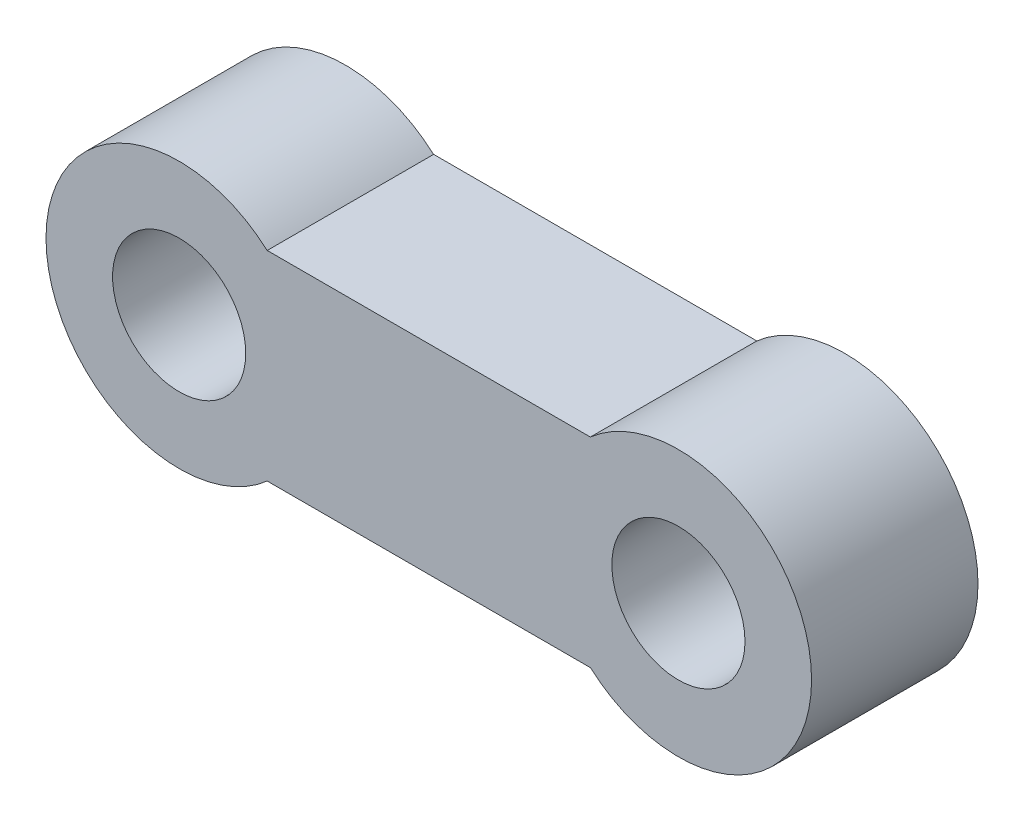
from build123d import *

# Parameters (mm, degrees)
SKETCH1_R           = 4
BOSS_EXTRUDE1_DEPTH = 10


with BuildPart() as part:
    # Sketch1 → Boss-Extrude1 (new body)
    with BuildSketch(Plane.XY):
        with BuildLine():
            Line((5.291502622, -6), (24.708497378, -6))
            ThreePointArc((24.708497378, -6), (38, 0), (24.708497378, 6))
            Line((24.708497378, 6), (5.291502622, 6))
            ThreePointArc((5.291502622, 6), (-8, 0), (5.291502622, -6))
        make_face()
        Circle(SKETCH1_R, mode=Mode.SUBTRACT)
        with Locations((30, 0)):
            Circle(SKETCH1_R, mode=Mode.SUBTRACT)
    extrude(amount=BOSS_EXTRUDE1_DEPTH)


solid = part.part
